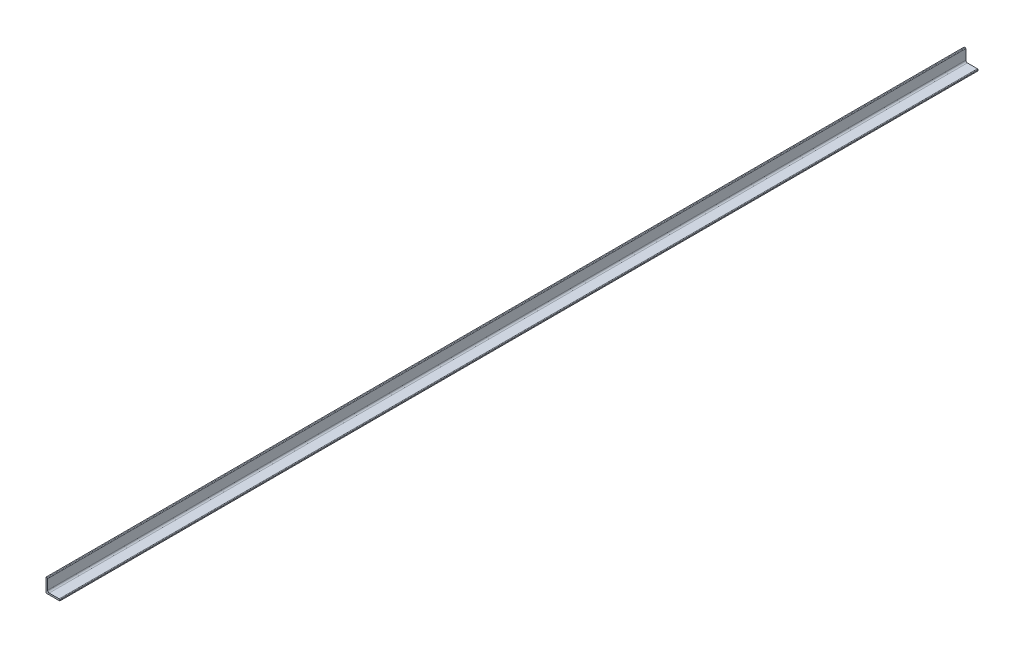
from build123d import *

# Parameters (mm, degrees)
BOSS_EXTRUDE1_DEPTH = 4660


with BuildPart() as part:
    # Sketch1 → Boss-Extrude1 (new body)
    with BuildSketch(Plane.XY):
        with BuildLine():
            Line((0, 70), (0, 0))
            Line((0, 0), (70, 0))
            Line((70, 0), (70, 5))
            ThreePointArc((70, 5), (69.121320344, 7.121320344), (67, 8))
            Line((67, 8), (16, 8))
            ThreePointArc((16, 8), (10.343145751, 10.343145751), (8, 16))
            Line((8, 16), (8, 67))
            ThreePointArc((8, 67), (7.121320344, 69.121320344), (5, 70))
            Line((5, 70), (0, 70))
        make_face()
    extrude(amount=BOSS_EXTRUDE1_DEPTH)


solid = part.part
